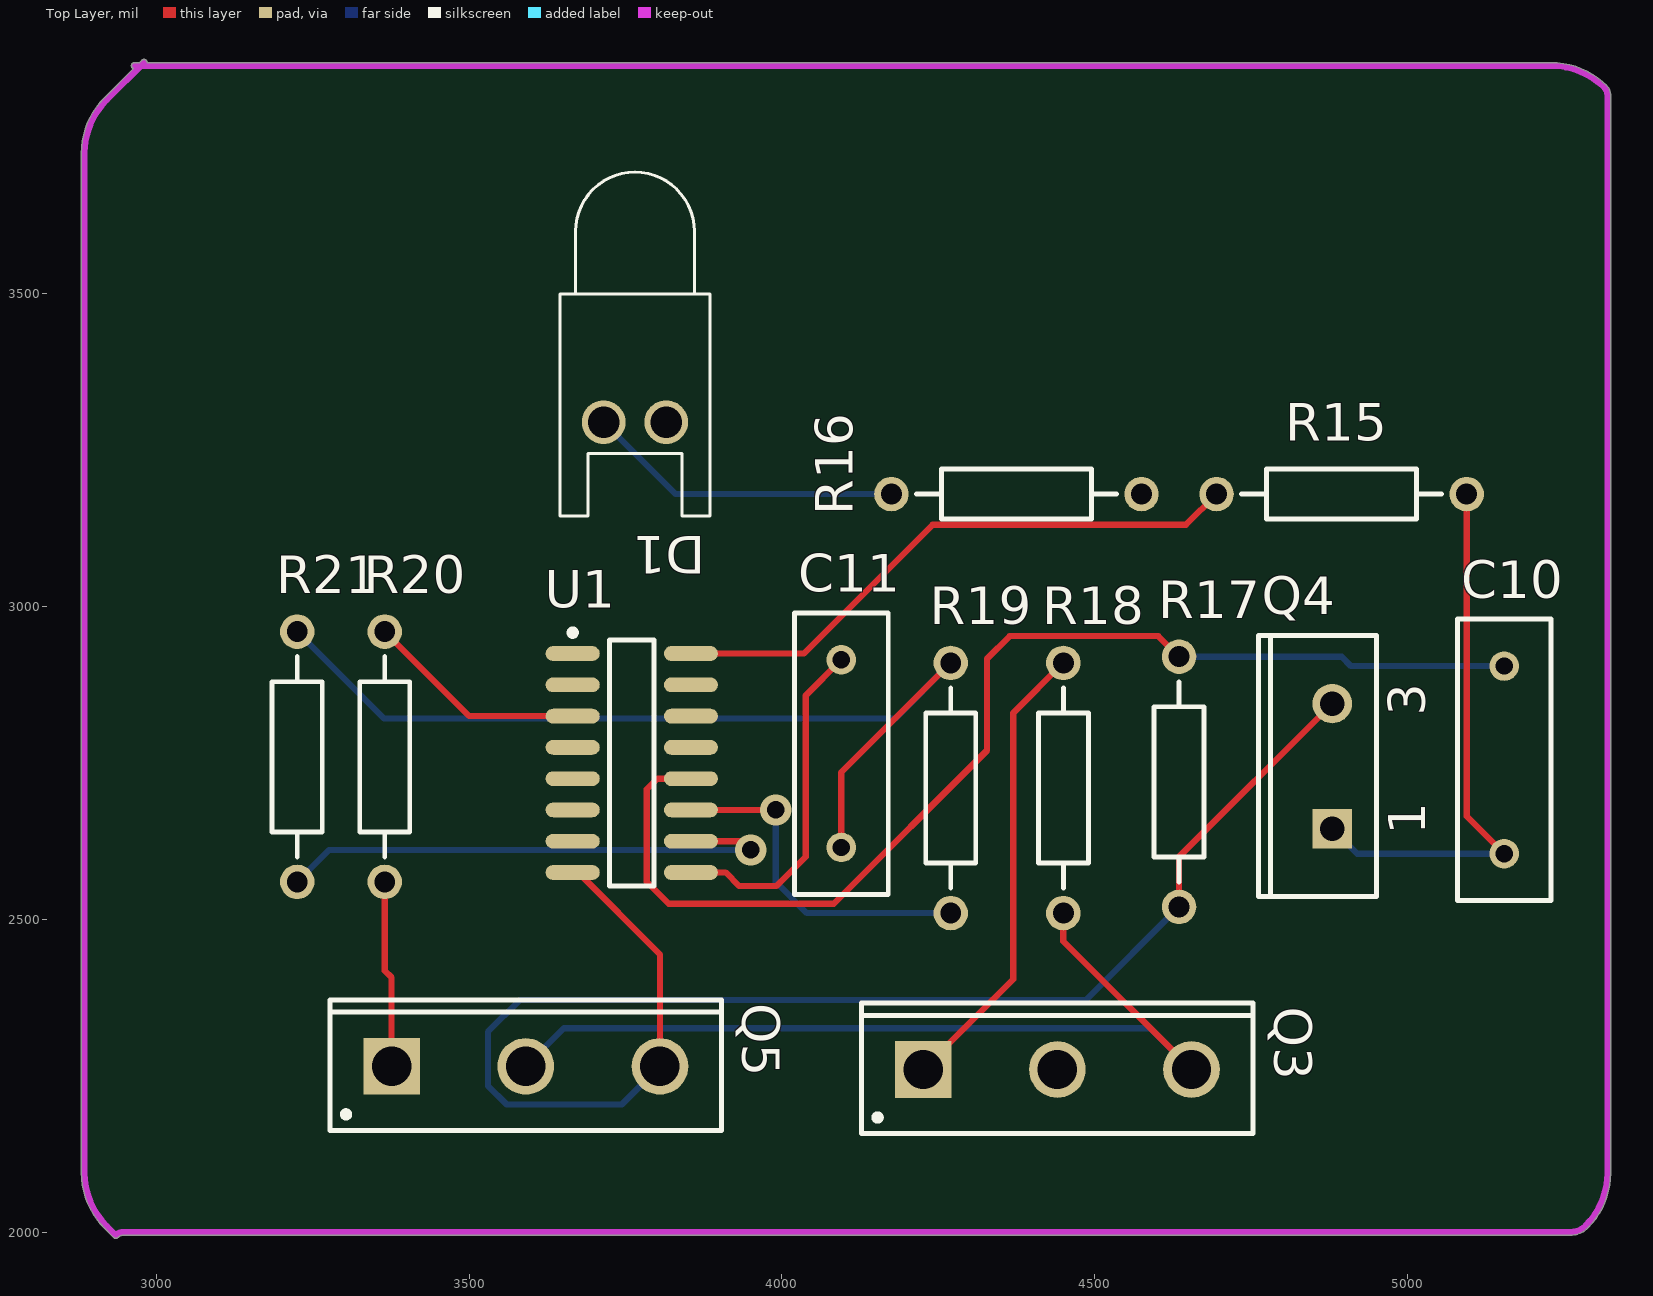
[diagram p0: Top Layer view]
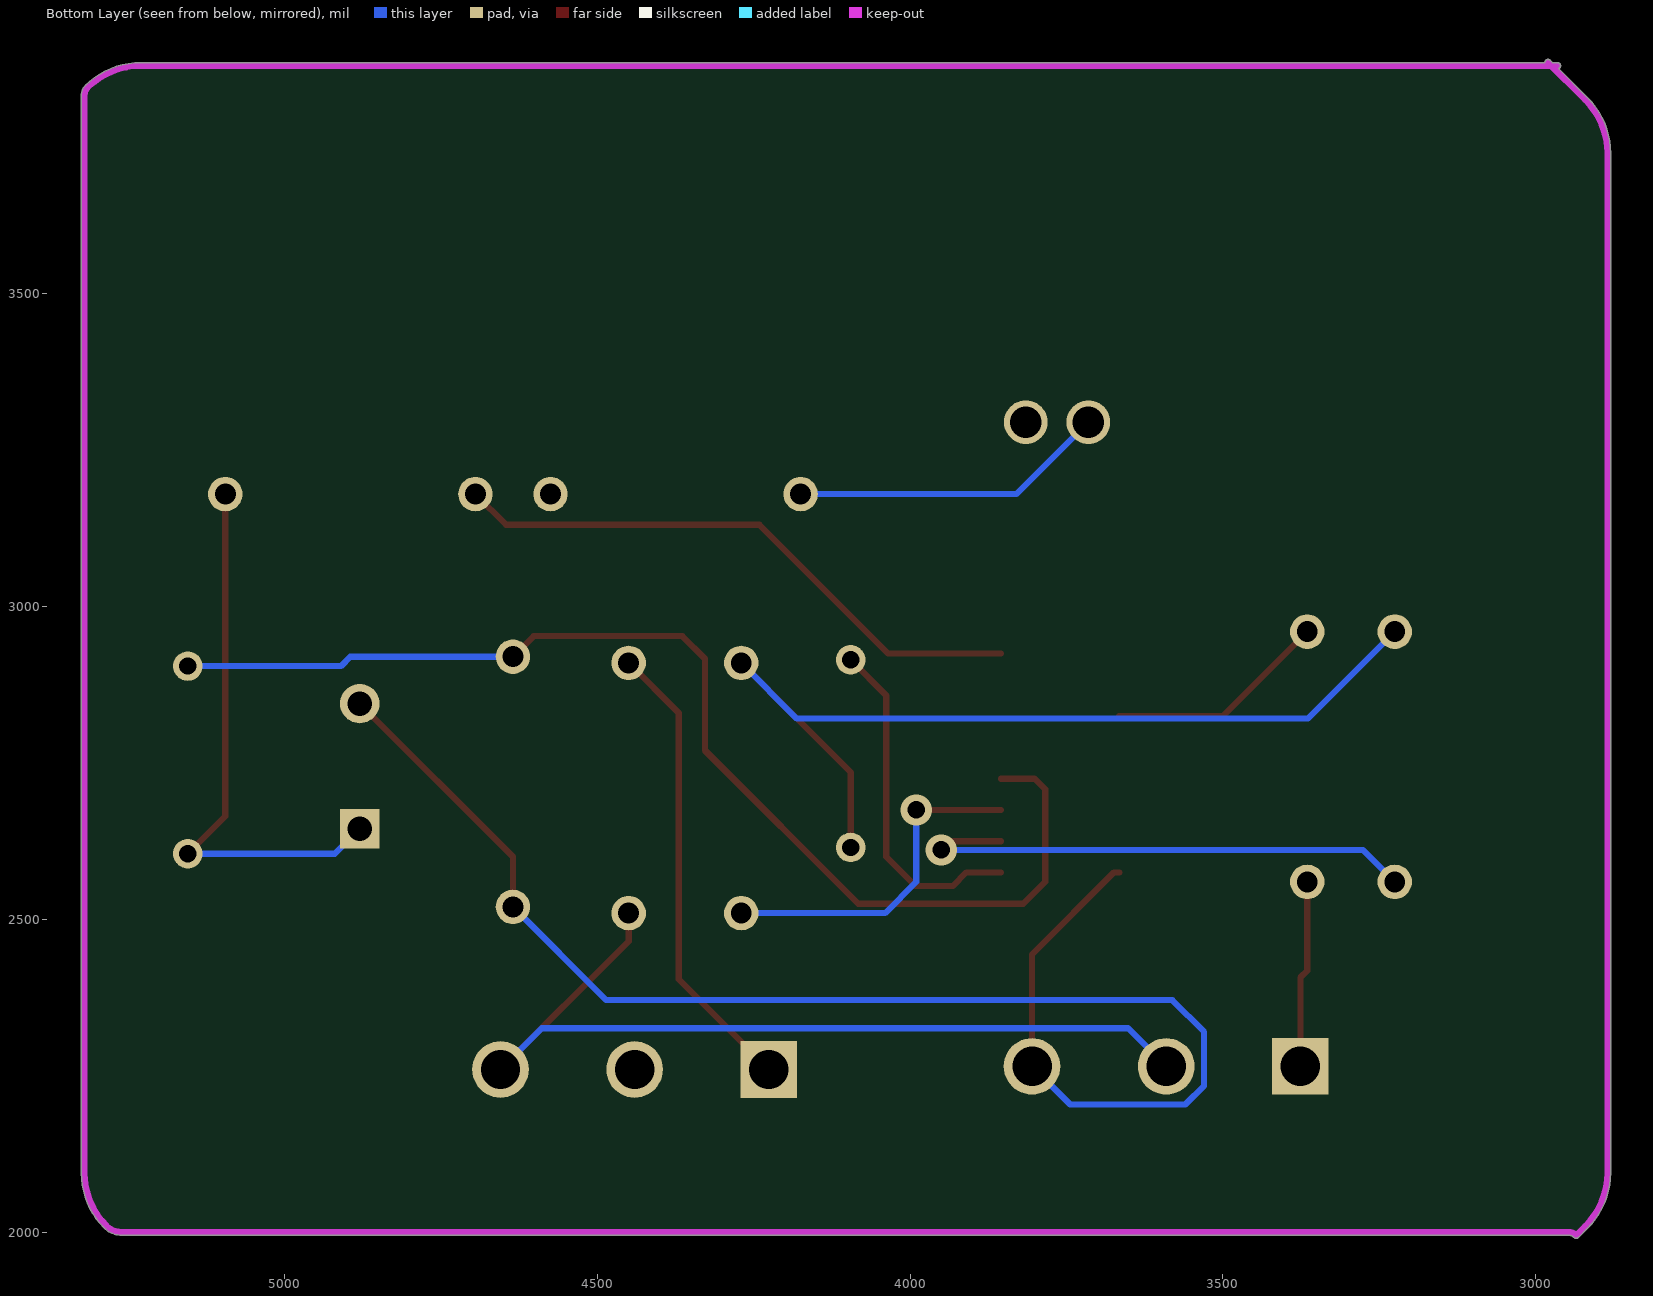
[diagram p1: Bottom Layer view, seen from below]
# Altium PCB MISC80684-4.PcbDoc
Units mil, origin at the board's own origin, x right, y up, seen from the top; angles counter-clockwise.
Board outline 2445.03 x 1885.02 mil, 2 copper layers (Top Layer, Bottom Layer); 14 components, 31 nets, 44 pads, 2 vias.

## Layer stack, top to bottom (the 12.6 mil dielectric is the usual default, probably not edited)
Top Solder: solder mask 0.4, Solder Resist, Dk 3.5
Top Layer: signal copper 1.4
Dielectric 1: dielectric 12.6, FR-4, Dk 4.8
Bottom Layer: signal copper 1.4
Bottom Solder: solder mask 0.4, Solder Resist, Dk 3.5

## Board outline
2916.81,2006.1 2931.45,1991.45 2931.44,1991.47 ccw(c2935,1995) 2938.55,1991.45 cw(c2947.07,1982.93) 2947.07,1994.98 5260.86,1994.98 ccw(c5260.86,2034.14) 5288.55,2006.45 ccw(c5200.5,2094.5) 5325.02,2094.5 5325.02,3818.43 ccw(c5304.14,3818.43) 5318.9,3833.19 ccw(c5230,3744.29) 5230,3870.01 2985.01,3870.01 ccw(c2980,3870) 2976.45,3873.55 2972.92,3870.01 2965,3870.01 ccw(c2965,3865) 2963.22,3860.31 2916.81,3813.9 cw(c2920.36,3810.36) 2916.83,3813.92 2916.81,3813.9 ccw(c3005.71,3725) 2879.99,3725 2879.99,2095 ccw(c3005.71,2095)

## Design rules (kind name [scope] priority, off if disabled: settings)
Clearance [All] p1: gap=10
PolygonConnect [All] p1: connectstyle=Relief reliefconductorwidth=10 reliefentries=4 polygonreliefangle="90 Angle" airgapwidth=10
RoutingVias [All] p1: holewidth=28 width=50 viastyle="Through Hole" minholewidth=28 minwidth=50 maxholewidth=28 maxwidth=50
SolderMaskExpansion [All] p1: expansion=4
Width [All] p1: maxlimit=10 minlimit=10 preferedwidth=10
30 further rules are at their usual default settings.

## Components (designator, comment, footprint, x,y, rotation, side; value= is the part's Value field where it differs from the comment)
C10 "Cap" RAD-0.3 5155,2755 r90 top
C11 "Cap" RAD-0.3 4095,2765 r90 top
D1 "LED0" LED-0 3765,3295 r180 top
Q3 "IRFP044N" TO-247AC 4440.43,2260 r0 top
Q4 "Photo NPN" TO-220_A 4880,2745 r90 top
Q5 "IRFP044N" TO-247AC 3590.43,2265 r0 top
R15 "Res2" AXIAL-0.4 4895,3180 r0 top
R16 "Res2" AXIAL-0.4 4375,3180 r180 top
R17 "Res2" AXIAL-0.4 4635,2720 r90 top
R18 "Res2" AXIAL-0.4 4450,2710 r90 top
R19 "Res2" AXIAL-0.4 4270,2710 r90 top
R20 "Res2" AXIAL-0.4 3365,2760 r90 top
R21 "Res2" AXIAL-0.4 3225,2760 r90 top
U1 "CD4060BCM" M16A_N 3760,2750 r0 top

## Footprints (in the part's own frame and the unit in brackets; to place one, negate y for a bottom-side part, rotate by r counter-clockwise, add the part's x,y. Pads: shape width x height; smd on the part's side, far side on the other; paste and mask are expansions set on the pad)
AXIAL-0.4 [mm] "Axial Device, Thru-Hole; 2 Leads; 0.4 in Pin Spacing"
  round 1.4 hole 0.85: 1(-5.08,0) 2(5.08,0)
  silkscreen extent -4.06,-1.02 4.06,1.02
LED-0 [mil] "LED; 2 Leads"
  round 70 hole 50: 1(50,0) 2(-50,0)
  silkscreen extent -120,-400 120,150
M16A_N [mm] "SOIC, 16-Leads, Body 9.9x3.9mm, Pitch 1.27mm, IPC Medium Density"
  oval 2.2x0.6 smd: 1(-2.4,4.445) 2(-2.4,3.175) 3(-2.4,1.905) 4(-2.4,0.635) 5(-2.4,-0.635) 6(-2.4,-1.905) 7(-2.4,-3.175) 8(-2.4,-4.445) 9(2.4,-4.445) 10(2.4,-3.175) 11(2.4,-1.905) 12(2.4,-0.635) 13(2.4,0.635) 14(2.4,1.905) 15(2.4,3.175) 16(2.4,4.445)
  silkscreen extent -2.52,-5 0.9,5.42, body extent -2,-5 2,5, height 1.75
RAD-0.3 [mm] "Radial Cap, Thru-Hole; 2 Leads; 0.3 in Pin Spacing"
  round 1.2 hole 0.7: 1(-3.81,0) 2(3.81,0)
  silkscreen extent -5.71,-1.91 5.71,1.91
TO-220_A [mm] "TO, Thru-Hole, Vertical, Heatsink Mounted; 3 In-Line Leads (1 Absent); Pitch 2.54 mm"
  rect 1.6x1.6 hole 1: 1(-2.54,0)
  round 1.6 hole 1: 3(2.54,0)
  silkscreen extent -5.3,-1.8 5.3,3
TO-247AC [mm] "SIP with Mounting Hole; 3 Leads; Body 20 x 15.6 x 5 mm (typ); Pitch 5.45 mm"
  rect 2.3x2.3 hole 1.6: 1(-5.45,0)
  round 2.3 hole 1.6: 2(0,0) 3(5.45,0)
  silkscreen extent -7.95,-2.6 7.95,2.7, body extent -7.95,-2.6 7.95,2.7, height 24.6

## Part data
C10 C11: "Capacitor"
D1: "Typical INFRARED GaAs LED"
Q3 Q5: "HEXFET Power MOSFET"
Q4: "NPN Phototransistor"
R15 R16 R17 R18 R19 R20 R21: "Resistor"
U1: "14-Stage Ripple Carry Binary Counter"

## Via types
v1: diameter 50, hole 28, Top Layer to Bottom Layer, 2 vias

## Nets (pads, with @x,y where several pads share a name; then routed paths per layer and width w, separated by ;. In a path a pad name is that pad's centre, name@x,y a point inside that pad or via, vN(x,y) a via of type N, cw(c..) or ccw(c..) an arc to the next point about the centre after c; other vN are vias at no path point)
+5: R15.1 U1.16 | length 946.1
  Top Layer w10: U1.16 4035,2925 4241,3131 4646,3131 R15.1
+12: Q3.1 R18.2 | length 742.8
  Top Layer w10: Q3.1 4370,2404.13 4370,2830 R18.2
GND: Q4.3 Q5.3 R17.1 U1.8 | length 2385.8
  Top Layer w10: U1.8 3674,2575 3805,2444 Q5.3 ; R17.1 4635,2600 Q4.3
  Bottom Layer w10: Q5.3 3744,2204 3560,2204 3530,2234 3530,2320 3581,2371 4486,2371 R17.1
NetC1_1: 
NetC2_1: 
NetC3_1: 
NetC3_2: 
NetC4_1: 
NetC5_1: 
NetC5_2: 
NetC6_2: 
NetC7_2: 
NetC8_1: 
NetC9_2: 
NetC10_1: C10.1 Q4.1 R15.2 | length 891.4
  Top Layer w10: R15.2 5095,2665 C10.1
  Bottom Layer w10: Q4.1 4920,2605 C10.1
NetC10_2: C10.2 R17.2 U1.12 | length 1894.3
  Top Layer w10: U1.12 3801,2725 3784,2708 3784,2560 3819,2525 4083,2525 4328,2770 4328,2917 4364,2953 4602,2953 R17.2
  Bottom Layer w10: R17.2 4895,2920 4910,2905 C10.2
NetC11_1: C11.1 R19.2 R21.2 | length 1506.9
  Top Layer w10: C11.1 4095,2735 R19.2
  Bottom Layer w10: R21.2 3364,2821 4181,2821 R19.2
NetC11_2: C11.2 U1.9 | length 550.6
  Top Layer w10: U1.9 3910,2575 3931.84,2553.16 3991.16,2553.16 4038,2600 4038,2858 C11.2
NetD1_1: D1.1 R16.2 | length 507.6
  Bottom Layer w10: D1.1 3830,3180 R16.2
NetD1_2: D1.2
NetQ1_1: 
NetQ2_2: 
NetQ3_3: Q3.3 Q5.2 R18.1 | length 1452.1
  Top Layer w10: R18.1 4450,2465 Q3.3
  Bottom Layer w10: Q5.2 3651.43,2326 4589,2326 Q3.3
NetQ5_1: Q5.1 R20.1 | length 299.5
  Top Layer w10: R20.1 3365,2417.87 3375.87,2407 Q5.1
NetR6_2: 
NetR8_3: 
NetR19_1: R19.1 U1.11 | length 551.2
  Top Layer w10: U1.11 v1(3990,2675)
  Bottom Layer w10: v1(3990,2675) 3990,2560 4040,2510 R19.1
NetR20_2: R20.2 U1.3 | length 356.4
  Top Layer w10: R20.2 3500,2825 U1.3
NetR21_1: R21.1 U1.10 | length 847.4
  Top Layer w10: U1.10 3936,2625 v1(3950,2611)
  Bottom Layer w10: R21.1 3276,2611 v1(3950,2611)
VCC: R16.1
VOUT: Q3.2
pads on no net: U1.1 U1.2 U1.4 U1.5 U1.6 U1.7 U1.13 U1.14 U1.15

## Keep-outs
Keep-Out Layer:
  lines w10: 2965,3865 5230,3865 cw(c5230,3744.29) 5315.36,3829.64 cw(c5304.14,3818.43) 5320,3818.43 5320,2094.5 cw(c5200.5,2094.5) 5285,2010 cw(c5260.86,2034.14) 5260.86,2000 2947.07,2000 ccw(c2947.07,1982.93) 2935,1995 2920.36,2009.64 cw(c3005.71,2095) 2885,2095 2885,3725 cw(c3005.71,3725) 2920.36,3810.36 2980,3870